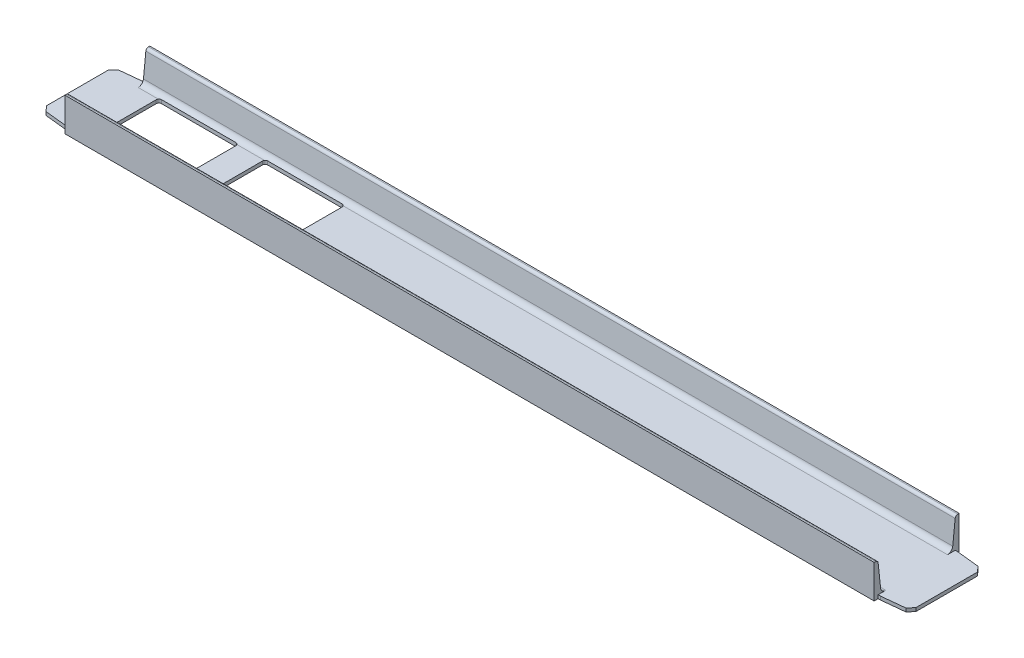
SolidWorks part; units mm, degrees
material "Q235B"
ref_plane "前视基准面" through (0, 0, 0) normal (0, 0, 1) x (1, 0, 0)
ref_plane "上视基准面" through (0, 0, 0) normal (0, 1, 0) x (1, 0, 0)
ref_plane "右视基准面" through (0, 0, 0) normal (1, 0, 0) x (0, 0, -1)
other "Configuration Table"
sketch "草图1" plane through (0, 0, 0) normal (0, 0, 1) x (1, 0, 0)
  line L0 (-818.5, 0) -> (818.5, 0)
  point P3 (0, 0)
  dimension "D1" = 1637
other "Gbt706-2008 热轧槽钢 16A(1)"
ref_plane "基准面1" through (-818.5, 0, 0) normal (1, 0, 0) x (0, 1, 0)
sketch "Sketch12" plane through (-818.5, 0, 0) normal (1, 0, 0) x (0, 1, 0)
  line L0 (63, 160) -> (0, 160)
  line L1 (63, 0) -> (0, 0)
  line L2 (0, 160) -> (0, 0)
  line L3 (-9.5694, 80) -> (49.7414, 80) construction
  line L4 (6.5, 138.0268) -> (6.5, 21.9732)
  line L5 (63, 0) -> (63, 2.5288)
  line L6 (63, 160) -> (63, 157.4712)
  line L7 (15.4547, 12.028) -> (58.5226, 7.5014)
  line L17 (15.4547, 147.972) -> (58.5226, 152.4986)
  arc A0 (58.5226, 152.4986) -> (63, 157.4712) centre (58, 157.4712) ccw
  arc A1 (58.5226, 7.5014) -> (63, 2.5288) centre (58, 2.5288) cw
  arc A2 (6.5, 21.9732) -> (15.4547, 12.028) centre (16.5, 21.9732) ccw
  arc A10 (6.5, 138.0268) -> (15.4547, 147.972) centre (16.5, 138.0268) cw
  point P6 (0, 0)
  point P8 (0, 80)
  point P9 (6.5, 25.8841)
  point P10 (31.5, 160)
  point P13 (63, 152.9692)
  point P14 (34.75, 150)
  point P19 (6.5, 80)
sketch "草图2" plane through (0, 0, 0) normal (0, -1, 0) x (1, 0, 0)
  line L0 (762, -5) -> (762, 7.5014)
  line L3 (-766.4774, 7.5014) -> (766.4774, 7.5014) construction
  line L4 (762, 7.5014) -> (766.4774, 7.5014)
  line L5 (766.4774, 7.5014) -> (809.5453, 12.028)
  line L6 (809.5453, 12.028) -> (818.5, 21.9732)
  line L7 (818.5, 21.9732) -> (818.5, 138.0268)
  line L8 (818.5, 138.0268) -> (809.5453, 147.972)
  line L9 (809.5453, 147.972) -> (766.4774, 152.4986)
  line L10 (766.4774, 152.4986) -> (762, 152.4986)
  line L11 (-766.4774, 152.4986) -> (766.4774, 152.4986) construction
  line L12 (762, 152.4986) -> (762, 165)
  line L14 (762, 165) -> (828.5, 165)
  line L15 (828.5, 165) -> (828.5, -5)
  line L16 (828.5, -5) -> (762, -5)
  line L18 (818.5, 0) -> (-818.5, 0) construction
  line L19 (818.5, 160) -> (-818.5, 160) construction
  line L20 (818.5, 160) -> (818.5, 0) construction
  dimension "D1" = 5
  dimension "D2" = 5
  dimension "D3" = 10
  dimension "D4" = 56.5
extrude "切除-拉伸1" cut sketch "草图2" against normal through all
sketch "草图3" plane through (0, 0, 0) normal (0, -1, 0) x (1, 0, 0)
  line L0 (-762, 0) -> (-762, 7.5014)
  line L1 (762, 0) -> (-818.5, 0) construction
  line L2 (-762, 2.5288) -> (-762, 0) construction
  line L3 (-766.4774, 7.5014) -> (766.4774, 7.5014) construction
  line L4 (-762, 7.5014) -> (-766.4774, 7.5014)
  line L5 (-766.4774, 7.5014) -> (-809.5453, 12.028)
  line L6 (-809.5453, 12.028) -> (-818.5, 21.9732)
  line L7 (-818.5, 160) -> (-818.5, 0) construction
  line L8 (-818.5, 21.9732) -> (818.5, 21.9732) construction
  line L9 (-818.5, 21.9732) -> (-818.5, 138.0268)
  line L10 (-818.5, 138.0268) -> (-809.5453, 147.972)
  line L11 (-809.5453, 147.972) -> (-766.4774, 152.4986)
  line L12 (-766.4774, 152.4986) -> (-762, 152.4986)
  line L13 (-766.4774, 152.4986) -> (766.4774, 152.4986) construction
  line L14 (-762, 152.4986) -> (-762, 165)
  line L15 (-762, 165) -> (-838.5, 165)
  line L16 (-838.5, 165) -> (-838.5, -5)
  line L17 (-838.5, -5) -> (-762, -5)
  line L18 (-762, -5) -> (-762, 0)
  line L19 (762, 160) -> (-818.5, 160) construction
  dimension "D1" = 20
  dimension "D2" = 5
  dimension "D3" = 5
extrude "切除-拉伸2" cut sketch "草图3" against normal through all
sketch "草图4" plane through (0, 0, 152.4986) normal (0, 0, 1) x (1, 0, 0)
  line L0 (818.5, 0) -> (818.5, 6.5) construction
  line L1 (818.5, 6.5) -> (762, 6.5)
  line L2 (818.5, 6.5) -> (818.5, 63)
  line L3 (818.5, 63) -> (762, 63)
  line L4 (762, 6.5) -> (762, 63)
  ellipse E0 centre (818.5, 16.5) end of major axis (818.5, 6.5) minor radius 9.004 (809.5453, 15.4547) -> (818.5, 6.5) ccw construction
extrude "切除-拉伸3" cut sketch "草图4" against normal through all
sketch "草图5" plane through (0, 0, 152.4986) normal (0, 0, 1) x (1, 0, 0)
  line L1 (-818.5, 6.5) -> (-762, 6.5)
  line L2 (-818.5, 6.5) -> (-818.5, 63)
  line L3 (-818.5, 63) -> (-762, 63)
  line L4 (-762, 6.5) -> (-762, 63)
extrude "切除-拉伸4" cut sketch "草图5" against normal through all
sketch "草图6" plane through (0, 0, 0) normal (0, -1, 0) x (1, 0, 0)
  line L0 (-772.2929, 0) -> (-107.7071, 0) construction
  line L1 (-580, 20) -> (-720, 20)
  line L2 (-575, 25) -> (-575, 105)
  line L3 (-580, 110) -> (-720, 110)
  line L4 (-725, 25) -> (-725, 105)
  line L5 (762, 160) -> (-762, 160) construction
  line L6 (-825, 85) -> (-825, -1855) construction
  line L7 (-375, 25) -> (-375, 105)
  line L8 (-380, 20) -> (-520, 20)
  line L9 (-525, 25) -> (-525, 105)
  line L10 (-380, 110) -> (-520, 110)
  line L11 (-575, 25) -> (-375, 25) construction
  arc A0 (-720, 110) -> (-725, 105) centre (-720, 105) ccw
  arc A1 (-580, 110) -> (-575, 105) centre (-580, 105) cw
  arc A2 (-725, 25) -> (-720, 20) centre (-720, 25) ccw
  arc A3 (-580, 20) -> (-575, 25) centre (-580, 25) ccw
  arc A4 (-380, 20) -> (-375, 25) centre (-380, 25) ccw
  arc A5 (-525, 25) -> (-520, 20) centre (-520, 25) ccw
  arc A6 (-520, 110) -> (-525, 105) centre (-520, 105) ccw
  arc A7 (-380, 110) -> (-375, 105) centre (-380, 105) cw
  point P16 (-725, 20)
  point P19 (-575, 20)
  dimension "D5" = 5
  dimension "D1" = 20
  dimension "D2" = 50
  dimension "D3" = 100
  dimension "D4" = 150
  dimension "D7" = 200
  dimension "D6" = 2
extrude "切除-拉伸5" cut sketch "草图6" against normal up to next
equation "\"RI@Sketch12\"= \"D1@Sketch12\""
equation "\"D3@Sketch12\"=  ( \"BF@Sketch12\" - \"D6@Sketch12\" )  / 2"
